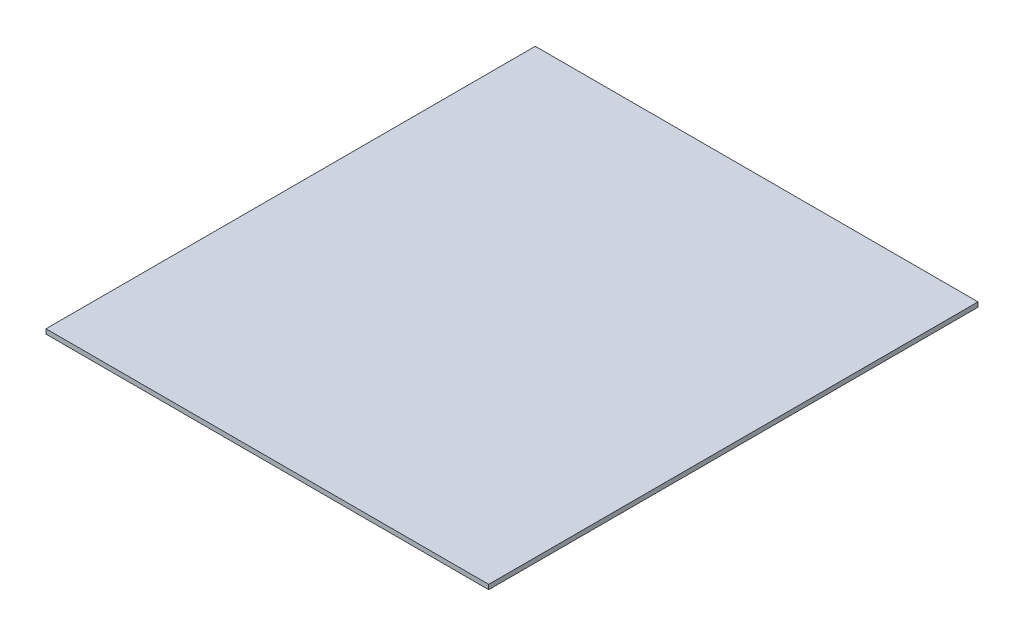
SolidWorks part; units mm, degrees
material "Q235"
ref_plane "Front Plane" through (0, 0, 0) normal (0, 0, 1) x (1, 0, 0)
ref_plane "Top Plane" through (0, 0, 0) normal (0, 1, 0) x (1, 0, 0)
ref_plane "Right Plane" through (0, 0, 0) normal (1, 0, 0) x (0, 0, -1)
sketch "Sketch1" plane through (0, 0, 0) normal (0, 1, 0) x (1, 0, 0)
  line L1 (-190, 210) -> (190, 210)
  line L2 (-190, 210) -> (-190, -210)
  line L3 (-190, -210) -> (190, -210)
  line L4 (190, 210) -> (190, -210)
  line L5 (-190, 210) -> (190, -210) construction
  line L6 (-190, -210) -> (190, 210) construction
  point P0 (0, 0)
  dimension "D1" = 420
  dimension "D2" = 380
extrude "Boss-Extrude1" add sketch "Sketch1" along normal blind 4
sketch "Sketch2" plane through (0, 4, 0) normal (0, 1, 0) x (1, 0, 0)
  line L0 (0, 0) -> (-190, 0) construction
  line L1 (-190, 210) -> (-140, 210)
  line L2 (-190, 210) -> (-190, 160)
  line L3 (-190, 160) -> (-140, 160)
  line L4 (-140, 210) -> (-140, 160)
  line L5 (-190, 210) -> (-190, -210) construction
  line L6 (-140, -210) -> (-140, -160)
  line L7 (-190, -160) -> (-140, -160)
  line L8 (-190, -210) -> (-190, -160)
  line L9 (-190, -210) -> (-140, -210)
  dimension "D1" = 50
  dimension "D2" = 50
extrude "Cut-Extrude1" [suppressed] cut sketch "Sketch2" against normal blind 10
